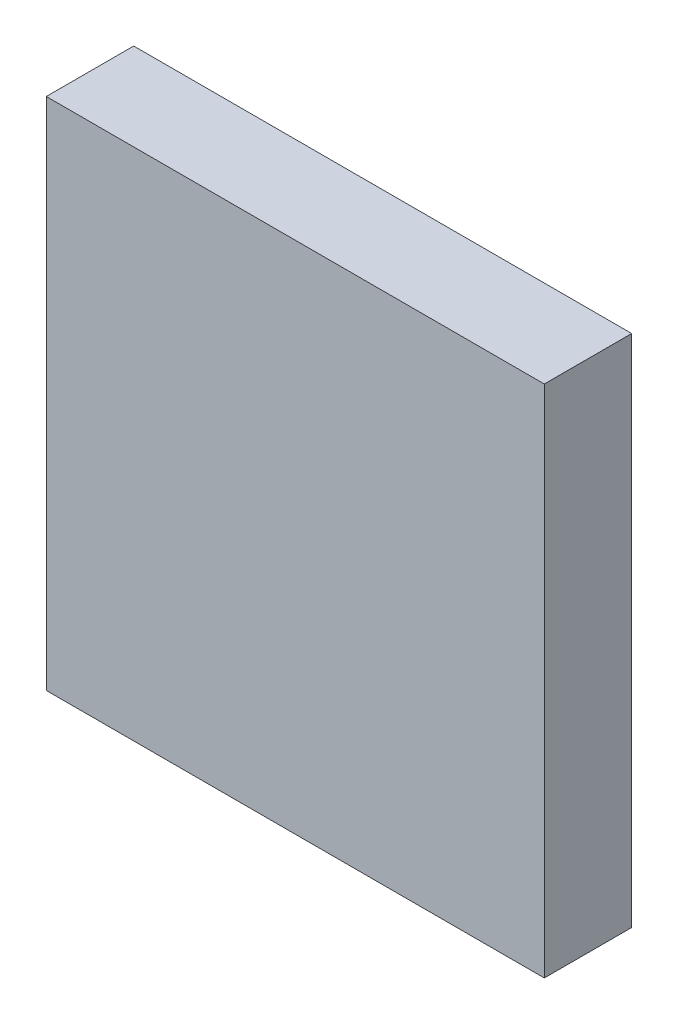
from build123d import *

# Parameters (mm, degrees)
SKETCH_1_W      = 56.968712564
SKETCH_1_H      = 58.84975496
EXTRUDE_1_DEPTH = 10


with BuildPart() as part:
    # 草图1 → 凸台-拉伸1 (new body)
    with BuildSketch(Plane.XY):
        Rectangle(SKETCH_1_W, SKETCH_1_H)
    extrude(amount=-EXTRUDE_1_DEPTH)


solid = part.part
